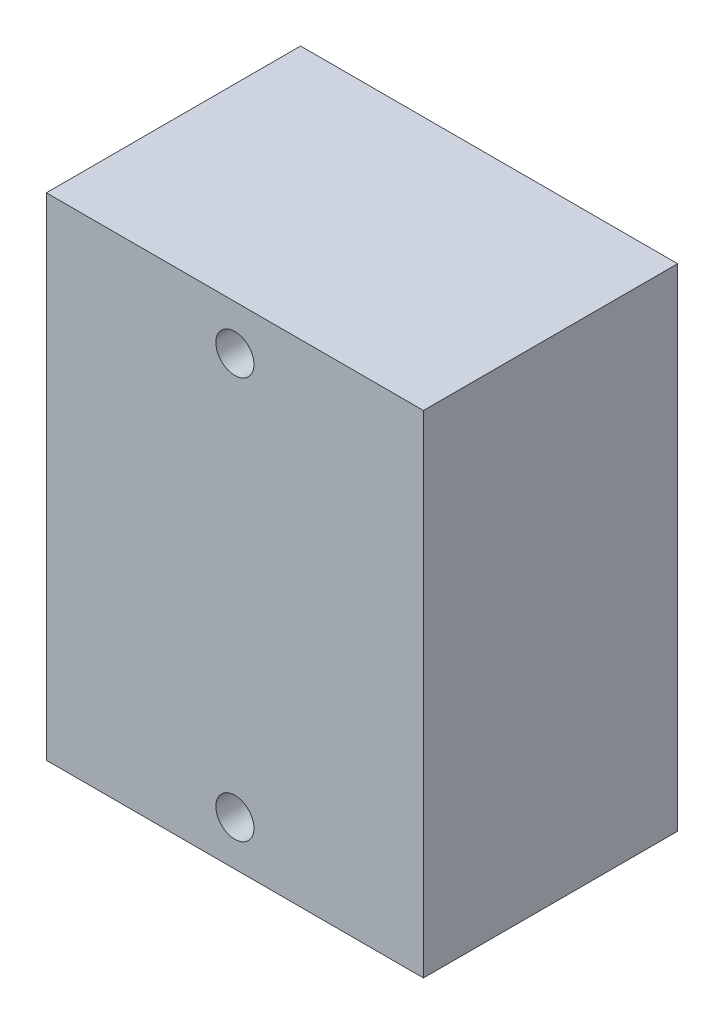
SolidWorks part; units mm, degrees
material "ABS"
ref_plane "前视基准面" through (0, 0, 0) normal (0, 0, 1) x (1, 0, 0)
ref_plane "上视基准面" through (0, 0, 0) normal (0, 1, 0) x (1, 0, 0)
ref_plane "右视基准面" through (0, 0, 0) normal (1, 0, 0) x (0, 0, -1)
sketch "草图1" plane through (0, 0, 0) normal (0, 0, 1) x (1, 0, 0)
  line L1 (-22.25, -29) -> (22.25, -29)
  line L2 (-22.25, -29) -> (-22.25, 29)
  line L3 (-22.25, 29) -> (22.25, 29)
  line L4 (22.25, -29) -> (22.25, 29)
  line L5 (0, 29) -> (0, -29) construction
  line L6 (-22.25, 0) -> (22.25, 0) construction
  circle A0 centre (0, 23.7) radius 2.25
  circle A1 centre (0, -23.7) radius 2.25
  point P0 (0, 0)
  dimension "D3" = 4.5
  dimension "D4" = 47.4
  dimension "D5" = 23.7
  dimension "D1" = 44.5
  dimension "D2" = 58
extrude "凸台-拉伸1" add sketch "草图1" along normal blind 30
